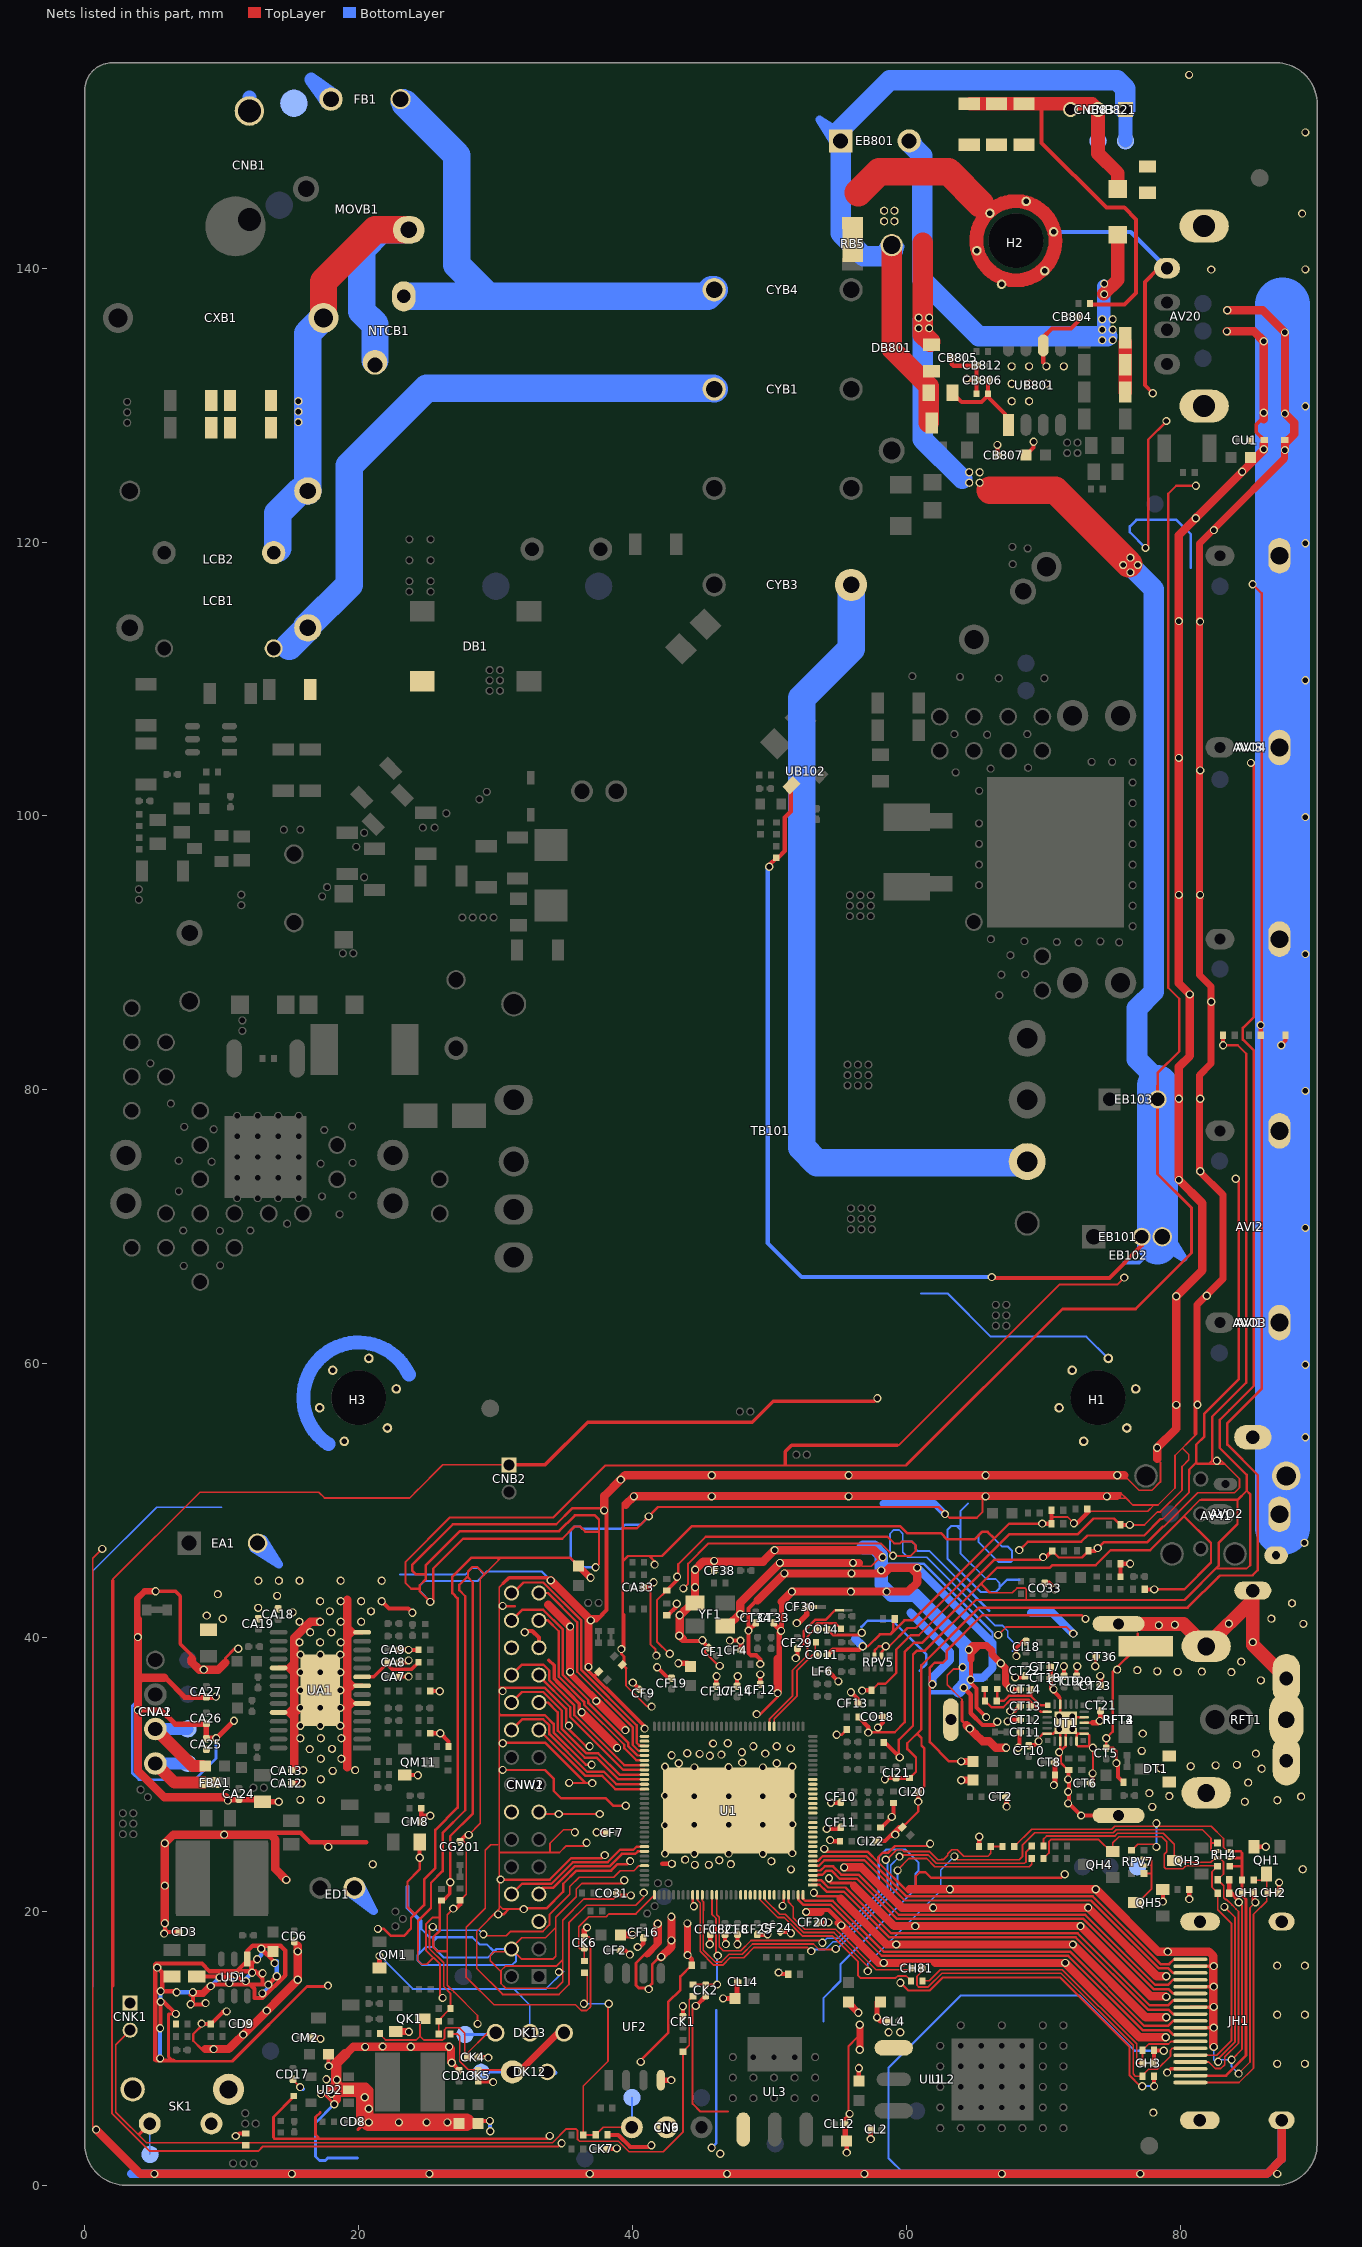
[diagram p0: the nets of this part, all layers, seen from the top]
# Altium PCB MISC116569.PcbDoc (part 10 of 15)
Units mm, origin at the board's own origin, x right, y up, seen from the top; angles counter-clockwise.
Board outline 90 x 155 mm, 2 copper layers (TopLayer, BottomLayer), stack 1.571 mm thick; 527 components, 277 nets, 2450 pads, 649 vias.

## Via types
v1: diameter 0.6, hole 0.4, TopLayer to BottomLayer, tented both sides, 649 vias

## Nets (pads, with @x,y where several pads share a name; then routed paths per layer and width w, separated by ;. In a path a pad name is that pad's centre, name@x,y a point inside that pad or via, vN(x,y) a via of type N, cw(c..) or ccw(c..) an arc to the next point about the centre after c; other vN are vias at no path point) (continued)
GND: (continued)
  BottomLayer w0.254: 23.546,21.78 23.546,20.255 24.385,19.416 24.385,16.989 ; v1(79.039,8.223) v1@79.039,8.295 ; v1@82.431,14.531 v1(82.456,14.506) ; v1(82.456,16.004) v1@82.456,16.035
  BottomLayer w0.3: v1(49.987,96.291) 49.873,96.178 49.873,68.803 52.357,66.319 v1(66.23,66.319) ; 75.946,67.373 76.98,67.373 EB102.2@78.349,68.742
  BottomLayer w0.305: v1@5.299,15.871 v1(5.299,15.89) ; v1(5.494,9.258) 5.498,9.262 v1(5.498,11.468) ; v1(5.532,14.16) 5.536,14.156 v1(5.536,13.399) ; v1(6.701,14.097) v1(7.895,14.097) ; v1@8.485,11.805 v1(8.526,11.805) ; v1(9.203,14.541) v1(9.838,15.176) ; v1(10.358,12.687) v1@10.473,12.687 ; v1(10.549,14.757) 10.652,14.655 10.652,14.975 v1(11.031,15.354) ; v1(11.755,14.91) 11.755,15.064 v1(12.214,15.523) ; v1(12.581,16.497) 12.917,16.834 12.917,17.241 v1(12.886,17.272) ; v1(12.975,14.008) 13.413,14.446 v1(13.413,14.649) ; v1(13.295,12.756) v1@13.324,12.756 ; v1(13.864,16.218) 14.022,16.377 v1(14.022,15.259) ; v1(15.548,15.009) 15.553,15.013 v1(15.553,17.069) ; v1@15.794,7.175 v1@15.938,7.031 ; v1(17.813,8.7) v1@17.851,8.661 ; v1(20.745,4.585) v1(20.745,5.577) ; 21.611,4.585 v1(22.944,4.585) ; v1(21.75,10.13) 21.77,10.109 v1(23.808,10.109) ; v1@23.63,39.091 v1(23.643,39.091) ; 24.201,4.585 v1(24.963,4.585) ; 25.725,4.585 v1(26.487,4.585) ; v1@25.903,36.068 v1(25.916,36.081) ; v1(26.805,8.943) v1@26.83,8.918 ; v1(29.591,4.699) 29.591,3.962 v1(29.616,3.937) ; v1@29.708,7.529 v1@29.737,7.529 ; DK12.K@34.334,8.238 DK12.K@34.359,8.213 ; v1(40.013,36.705) v1@40.089,36.629 ; v1(44.023,16.808) v1@44.1,16.731 ; v1@45.206,39.77 v1@45.238,39.77 ; v1(45.639,17.605) v1@45.664,17.63 ; v1@45.956,45.579 v1(45.956,45.593) ; v1@46.136,37.101 v1(46.136,37.169) ; v1@46.732,17.605 v1(46.824,17.605) ; v1@47.633,17.63 v1(47.658,17.605) ; v1@47.683,37.099 v1(47.683,37.169) ; v1@49.335,37.925 v1(49.335,38.064) ; v1@49.847,18.332 v1(49.863,18.332) ; v1(50.668,15.535) v1@50.757,15.623 ; v1@51.562,18.409 v1(51.567,18.404) ; v1@54.26,19.232 v1(54.3,19.192) ; v1(54.496,27.927) v1@54.514,27.927 ; v1(58.928,26.899) v1@58.928,26.924 ; v1(60.871,28.016) v1@60.884,28.003 ; 64.448,39.461 64.498,39.461 ; v1(66.632,33.848) v1@66.657,33.873 ; v1@67.584,36.274 v1@67.648,36.274 ; v1@70.738,36.219 v1(70.754,36.219) ; H2.4@70.75,142.654 76.386,142.654 AV20.4@79.04,140 ; v1(71.505,37.897) v1@71.533,37.925 ; v1@72.436,37.899 v1@72.449,37.887 ; v1@72.474,37.887 v1(72.487,37.899) ; v1@76.309,48.212 v1(76.322,48.224) ; v1(78.735,20.716) v1@78.748,20.729 ; v1(80.653,20.894) v1@80.653,20.97 ; v1(83.129,83.251) v1@83.155,83.251 ; v1(84.277,20.663) v1@84.346,20.663 ; v1(85.491,20.653) v1@85.504,20.665 ; v1(85.872,84.724) v1@85.897,84.7
  BottomLayer w0.33: 61.85,35.986 63.508,35.986
  BottomLayer w0.381: v1@9.58,35.602 v1(9.58,35.689) ; v1@15.799,29.362 v1(15.862,29.362) ; v1@21.509,16.726 v1(21.522,16.739) ; v1@36.588,18.821 v1(36.68,18.821) ; v1(46.617,13.642) v1@46.655,13.68 ; v1@52.002,41.036 v1(52.002,41.049) ; v1(67.318,27.648) v1@67.318,27.711 ; v1(74.155,37.189) v1@74.176,37.169
  BottomLayer w0.508: v1@23.655,11.214 v1(23.668,11.214) ; v1(45.779,2.743) v1@45.782,2.743 ; 58.306,49.784 62.05,49.784 v1(62.822,49.012)
  BottomLayer w0.61: 3.373,0.826 47.353,0.826 ; 47.816,0.826 47.353,0.826 ; 56.261,39.914 v1(56.815,39.36) ; v1@58.166,45.083 60.803,45.083 66.289,39.596 66.289,37.782 65.561,37.053 64.593,37.053 64.359,37.287 ; 60.308,41.806 63.173,38.941 63.173,38.356 61.908,37.091 v1(61.908,36.591) ; 69.121,41.819 70.65,41.819 v1(72.182,40.287) ; JH1.21@87.409,4.75 87.409,1.907 86.327,0.826 47.353,0.826
  BottomLayer w1: pad.VIA5@74.417,135.255 pad.VIA5@74.417,138.659
  BottomLayer w1.016: 17.786,54.12 cw(c20,57.502) 23.667,59.204 ; 56.87,46.581 57.623,46.581 58.166,46.039 58.166,43.867 58.927,43.106 60.624,43.106 63.803,39.927 ; 63.826,36.136 64.359,36.669 64.359,39.372 63.803,39.927 ; 64.185,39.545 63.803,39.927
  BottomLayer w1.5: EB801.2@60.242,149.119 61.149,148.212 61.149,144.412 ; 61.149,139.201 61.149,140.437 ; 61.149,145.907 61.149,144.412 ; 61.209,136.195 61.209,127.495 64.079,124.625 ; 74.658,135.026 65.291,135.026 61.149,139.168 61.149,140.437 ; 76.233,118.402 78.067,116.568 78.067,87.165 76.843,85.941 76.843,82.233 78.177,80.898 78.177,80.675 78.443,80.409 ; 61.149,140.437 61.149,144.412
  BottomLayer w2: CYB3.2@55.964,116.874 55.964,112.212 52.362,108.61 52.362,75.789 53.473,74.678 TB101.8@68.643,74.678
  BottomLayer w3: EB102.2@78.349,68.742 78.349,80.315
  BottomLayer w4: AVO3.2@87.479,48.012 87.479,54.892 ; 87.479,52.9 87.479,54.892 ; 87.479,137.34 87.479,54.892
  other v1: 5.088,0.826 15.126,0.826 25.172,0.826 36.881,0.826 46.901,0.826 56.939,0.826 66.98,0.826 77.077,0.826 87.084,0.826 46.414,2.294 29.813,7.529 58.701,11.178 59.56,11.178 78.983,12.264 55.248,18.976 42.845,19.599 30.201,19.773 44.488,20.372 44.524,24.207 49.524,24.207 42.374,24.219 47.012,24.219 51.674,24.257 42.374,26.282 44.524,26.307 49.524,26.307 47.012,26.319 51.674,26.357 71.814,27.879 44.524,28.407 47.012,28.419 49.524,28.407 42.374,28.457 51.674,28.457 71.814,28.743 71.814,29.632 44.524,30.507 49.524,30.507 47.012,30.519 42.374,30.557 51.674,30.557 50.533,30.811 48.01,30.866 45.656,31.37 42.858,31.394 46.495,31.446 44.894,31.501 49.695,31.522 44.005,31.548 51.549,31.903 48.831,32.056 77.262,32.982 71.157,33.297 72.107,33.297 15.754,33.554 17.204,33.554 18.654,33.554 71.157,34.247 72.107,34.247 15.754,34.854 17.204,34.854 18.654,34.854 15.754,36.154 17.204,36.154 18.654,36.154 15.754,37.454 17.204,37.454 18.654,37.454 8.687,37.655 15.754,38.754 17.204,38.754 18.654,38.754 10.071,41.377 8.903,41.605 36.939,44.364 56.104,45.443 55.784,50.305 45.783,51.854 55.784,51.854 65.784,51.854 89.147,54.625 89.147,59.913 89.147,69.913 89.147,79.913 82.261,86.436 89.147,89.913 81.448,94.234 89.147,99.913 79.904,104.234 89.147,109.913 81.453,114.191 79.904,114.234 89.147,119.913 86.101,126.771 89.147,129.913 82.271,139.9 89.147,139.913 88.9,143.993 89.147,149.913 80.645,154.12
GVDD: CA8.2@22.114,38.177 CA8.2@22.289,38.177 RA10.1 UA1.9 | length 5
  TopLayer w0.254: UA1.9@20.254,37.129 21.092,37.129 22.114,38.151 22.114,37.993 22.409,37.698 23.888,37.698 24.379,38.189 RA10.1@24.379,38.195
HDMI_A_0N_IN_IC: JH1.9 U1.1 | length 32.3
  TopLayer w0.178: U1.1@53.075,21.932 U1.1@53.175,21.932 53.672,21.932 54.166,21.438 55.425,21.438 58.764,18.1 72.376,18.1 77.649,12.827 79.154,12.827 ; 78.392,12.827 79.154,12.827 ; JH1.9@80.742,12.5 79.481,12.5 79.154,12.827
HDMI_A_0P_IN_IC: JH1.7 U1.2 | length 31.5
  TopLayer w0.178: U1.2@53.175,22.282 53.753,22.282 54.292,21.743 55.551,21.743 58.89,18.405 72.502,18.405 77.775,13.131 79.103,13.131 79.472,13.5 JH1.7@80.742,13.5
HDMI_A_1N_IN_IC: JH1.6 U1.3 | length 31.4
  TopLayer w0.178: U1.3@53.175,22.632 53.526,22.632 53.571,22.678 53.868,22.678 54.167,22.977 54.522,22.977 55.12,22.378 56.389,22.378 59.321,19.446 72.933,19.446 78.053,14.327 79.154,14.327 79.481,14 JH1.6@80.742,14
HDMI_A_1P_IN_IC: JH1.4 U1.4 | length 31.4
  TopLayer w0.178: U1.4@53.175,22.982 53.741,22.982 54.041,23.282 54.648,23.282 55.247,22.683 56.515,22.683 59.448,19.751 73.059,19.751 78.179,14.631 79.103,14.631 79.472,15 JH1.4@80.742,15
HDMI_A_2N_IN_IC: JH1.3 U1.5 | length 31.1
  TopLayer w0.178: U1.5@53.175,23.332 53.619,23.332 54.019,23.732 56.939,23.732 59.879,20.792 73.491,20.792 78.446,15.837 79.144,15.837 79.481,15.5 JH1.3@80.742,15.5
HDMI_A_2P_IN_IC: JH1.1 U1.6 | length 31.1
  TopLayer w0.178: U1.6@53.175,23.682 53.538,23.682 53.893,24.037 57.065,24.037 60.005,21.097 73.617,21.097 78.572,16.142 79.19,16.142 79.548,16.5 JH1.1@80.742,16.5
HDMI_A_5V: CH1.1 JH1.18 RH3.2 RH4.1 RH4.3 RH4.5 RH81.2 RPV7.1 | length 44.4
  TopLayer w0.127: RH81.2@67.881,24.74 69.145,26.003 75.002,26.003 75.214,26.215 82.271,26.215 83.163,25.323 83.163,24.684 83.453,24.394 RH4.5@83.622,24.394 ; RPV7.1@76.451,24.458 76.891,24.898 78.198,24.898 78.265,24.831 v1(78.265,24.704) ; v1@78.252,26.418 v1(78.265,26.431)
  TopLayer w0.203: JH1.18@80.742,8 83.34,8 84.806,9.466 84.806,20.882 84.52,21.167 CH1.1@84.52,21.365 ; RH4.1@83.622,23.294 84.52,23.294 ; RH4.3@83.622,23.894 84.52,23.894 ; RH4.5@83.622,24.394 84.391,24.394 84.52,24.265 84.52,23.894 ; CH1.1@84.608,21.277 CH1.1@84.52,21.365 ; CH1.1@84.52,21.365 RH3.2@84.52,22.278 84.52,23.294 ; 84.52,23.294 84.52,23.894
  BottomLayer w0.127: v1(78.265,24.704) 78.265,25.479 ; 78.265,26.05 78.265,25.479 ; v1(78.265,26.431) 78.265,25.479
HDMI_A_CKN_IN_IC: JH1.12 U1.127 | length 33.1
  TopLayer w0.178: U1.127@52.099,21.207 52.099,20.854 52.48,20.473 54.487,20.473 58.206,16.754 71.818,16.754 77.245,11.327 79.154,11.327 79.481,11 JH1.12@80.742,11
HDMI_A_CKP_IN_IC: JH1.10 U1.128 | length 33.3
  TopLayer w0.178: U1.128@52.449,21.207 52.449,20.935 52.606,20.778 54.613,20.778 58.332,17.059 71.944,17.059 77.371,11.631 79.103,11.631 ; 78.392,11.631 79.103,11.631 ; JH1.10@80.742,12 79.472,12 79.103,11.631
HDMI_A_HPD_OUT: CH2.1 JH1.19 QH1.C RH3.1 | length 21.1
  TopLayer w0.127: JH1.19@80.742,7.5 84.297,7.5 85.352,8.554 85.352,19.776 86.317,20.742 QH1.C@86.317,22.735 QH1.C@86.59,22.461 ; RH3.1@85.37,22.278 QH1.C@86.408,22.278
HDMI_A_HPD_OUT_IC: RH4.6 RH4.8 U1.120 | length 44.4
  TopLayer w0.127: U1.120@49.649,21.207 49.698,21.157 49.698,20.829 50.743,19.784 51.168,19.784 52.504,18.448 54.716,18.448 57.188,15.976 v1(57.188,15.642) ; U1.120@49.649,21.207 U1.120@49.65,21.257 ; v1(63.513,24.016) 63.754,23.774 64.668,23.774 ; 63.856,23.774 64.668,23.774 ; RH4.6@82.722,24.394 82.334,24.394 82.245,24.483 82.245,24.996 ; RH4.8@82.722,24.994 82.72,24.996 82.245,24.996 ; 64.668,23.774 68.247,23.774 68.489,24.016 68.489,24.853 69.385,25.749 75.107,25.749 75.319,25.961 81.631,25.961 82.245,25.347 82.245,24.996
  BottomLayer w0.127: v1(57.188,15.642) 57.188,16.194 62.517,21.524 62.517,23.02 v1(63.513,24.016)
HDMI_A_SCL_IN: DH2.K JH1.15 QH4.E RH4.2 RH6.1 | length 34.3
  TopLayer w0.127: RH6.1@70.008,23.863 70.409,24.264 70.409,25.095 70.555,25.241 74.047,25.241 74.917,24.371 QH4.E@75.082,24.371 75.082,25.006 75.529,25.453 78.659,25.453 79.018,25.094 79.018,24.366 78.832,24.18 78.832,23.222 78.944,23.11 80.201,23.11 80.417,23.326 82.691,23.326 RH4.2@82.722,23.294 82.321,22.893 82.321,21.754 DH2.K@82.736,21.338 82.736,20.122 83.752,19.107 83.752,10.582 82.67,9.5 JH1.15@80.742,9.5
HDMI_A_SCL_IN_IC: RH6.2 U1.107 | length 33.4
  TopLayer w0.127: U1.107@45.099,21.207 45.1,20.785 45.183,20.702 45.183,20.064 ; 45.174,20.055 45.174,17.169 46.039,16.304 46.493,16.304 47.049,16.86 48.01,16.86 48.763,17.613 53.221,17.613 53.622,17.213 54.804,17.213 v1(54.851,17.26) ; v1@59.36,23.046 60.173,23.858 61.489,23.858 62.081,23.266 68.984,23.266 69.158,23.441 RH6.2@69.158,23.863
  BottomLayer w0.127: v1(54.851,17.26) 54.944,17.26 59.36,21.675 v1(59.36,22.987)
HDMI_A_SDA_IO: DH3.K JH1.16 QH3.C RH4.4 RH5.1 | length 34.4
  TopLayer w0.127: RH5.1@70.008,24.778 70.008,25.266 70.237,25.495 75.212,25.495 75.424,25.707 78.764,25.707 79.018,25.453 ; JH1.16@80.742,9 82.082,9 82.563,8.519 82.969,8.519 83.257,8.806 83.257,9.368 84.26,10.371 84.26,19.986 84.074,20.172 83.787,20.459 83.373,20.873 83.283,20.873 83.171,20.984 83.171,21.869 DH3.K@82.736,22.304 83.163,22.73 83.163,23.623 RH4.4@82.892,23.894 ; RH4.4@82.722,23.894 82.553,23.894 82.239,23.58 79.693,23.58 QH3.C@79.572,23.701 79.572,24.899 79.027,25.444 ; 79.018,25.453 79.027,25.444 ; 79.018,25.453 79.027,25.453 79.027,25.444
HDMI_A_SDA_IO_IC: RH5.2 U1.106 | length 34.9
  TopLayer w0.127: U1.106@44.749,21.207 44.75,20.812 44.954,20.607 44.954,20.159 ; U1.106@44.749,21.207 U1.106@44.759,21.198 ; 44.945,20.149 44.945,17.075 45.944,16.075 46.587,16.075 47.118,16.606 48.115,16.606 48.868,17.359 52.782,17.359 v1(53.047,17.094) ; v1(59.499,24.003) 59.609,24.112 61.595,24.112 62.187,23.52 68.628,23.52 68.743,23.635 68.743,24.362 RH5.2@69.158,24.778
  BottomLayer w0.127: v1@53.047,17.174 52.967,17.174 v1(53.047,17.094) 53.165,17.213 54.069,17.213 54.642,17.785 55.11,17.785 58.869,21.544 58.869,23.373 v1(59.499,24.003)
HDMI_ARC_OUT: CH81.1 DH81.K JH1.14 | length 27.3
  TopLayer w0.127: CH81.1@61.19,15.839 61.19,15.683 60.774,15.268 60.774,14.596 60.887,14.483 61.601,14.483 62.602,15.484 71.292,15.484 76.563,10.212 76.563,8.13 76.728,7.965 77.186,7.965 77.685,8.465 78.327,8.465 79.289,9.426 79.289,9.866 79.424,10 JH1.14@80.742,10
HDMI_ARC_OUT_IC: CH81.2@60.34,15.839 CH81.2@60.515,15.839 U1.125 | length 12
  TopLayer w0.127: U1.125@51.399,21.207 51.399,20.664 51.748,20.316 51.748,19.528 52.574,18.702 54.821,18.702 55.245,18.278 57.785,15.738 60.238,15.738 CH81.2@60.34,15.839
HDMI_B_0N_IN_IC: U1.9
HDMI_B_0P_IN_IC: U1.10
HDMI_B_1N_IN_IC: U1.11
HDMI_B_1P_IN_IC: U1.12
HDMI_B_2N_IN_IC: U1.13
HDMI_B_2P_IN_IC: U1.14
HDMI_B_CKN_IN_IC: U1.7
HDMI_B_CKP_IN_IC: U1.8
HDMI_B_HPD_OUT_IC: U1.121
HDMI_B_SCL_IN_IC: U1.116
HDMI_B_SDA_IO_IC: U1.115
HDMI_C_0N_IN_IC: U1.18
HDMI_C_0P_IN_IC: U1.19
HDMI_C_1N_IN_IC: U1.20
HDMI_C_1P_IN_IC: U1.21
HDMI_C_2N_IN_IC: U1.22
HDMI_C_2P_IN_IC: U1.23
HDMI_C_CKN_IN_IC: U1.16
HDMI_C_CKP_IN_IC: U1.17
HDMI_C_HPD_OUT_IC: U1.122
HDMI_C_SCL_IN_IC: U1.118
HDMI_C_SDA_IO_IC: U1.117
HDMI_CEC_IO: CH3.2@77.239,8.905 CH3.2@77.414,8.905 DH1.K JH1.13 RH83.2 | length 24.7
  TopLayer w0.127: RH83.2@61.19,14.925 61.669,14.925 62.481,15.738 71.397,15.738 76.817,10.317 76.817,8.981 76.894,8.905 CH3.2@77.239,8.905 77.239,9.841 DH1.K@77.243,9.845 77.709,10.311 79.144,10.311 79.333,10.5 JH1.13@80.742,10.5
HDMI_CEC_IO_IC: RH83.1 U1.119 | length 14.6
  TopLayer w0.127: U1.119@49.3,21.257 49.3,21.207 49.299,20.87 50.624,19.545 ; 50.631,19.552 51.076,19.552 52.435,18.194 54.611,18.194 56.473,16.332 56.473,16.296 ; 56.473,16.296 56.473,15.309 56.642,15.14 59.232,15.14 59.368,15.276 59.989,15.276 RH83.1@60.34,14.925
HDMI_DET: RH81.1 RH82.1 U1.110 | length 30.4
  TopLayer w0.127: U1.110@46.15,21.207 46.15,19.757 46.333,19.573 46.333,17.402 46.622,17.114 47.904,17.114 48.657,17.867 v1@53.702,17.867 ; v1@58.49,23.831 v1(58.49,23.773) 58.576,23.773 59.296,24.493 59.703,24.493 59.83,24.366 61.7,24.366 62.292,23.774 62.56,23.774 62.565,23.779 62.7,23.779 63.022,24.102 63.022,24.219 63.31,24.506 63.716,24.506 64.194,24.028 65.964,24.028 66.167,24.232 RH82.1@66.167,24.74 RH81.1@67.032,24.74
  BottomLayer w0.127: v1(53.866,17.703) 54.202,18.039 55.005,18.039 58.615,21.649 v1@58.615,23.648
I2C_EN: QH5.C RPV7.4 RPV7.6 RPV7.8 | length 5.4
  TopLayer w0.127: QH5.C@76.753,20.64 76.894,20.64 77.91,21.656 77.91,22.748 ; RPV7.8@77.351,22.758 77.9,22.758 77.91,22.748 ; RPV7.6@77.351,23.358 77.871,23.358 77.91,23.396 ; RPV7.4@77.351,23.858 77.778,23.858 77.91,23.726 77.91,23.396 ; 77.91,22.748 77.91,23.396
IF_N: CT13.1 RT10.1 RT12.2 UT1.14 | length 6.3
  TopLayer w0.178: RT12.2@65.711,35.407 RT10.1@65.711,36.263 ; RT12.2@65.75,35.368 66.216,34.902 67.077,34.902 67.619,35.444 68.948,35.444 69.82,34.572 UT1.14@70.282,34.572 ; CT13.1@68.933,34.978 CT13.1@69.108,34.978
IF_P: CT14.2@68.94,36.21 CT14.2@69.115,36.21 RT12.1 RT13.1 UT1.13 | length 5.5
  TopLayer w0.178: RT13.1@66.651,36.263 66.651,35.419 RT12.1@66.6,35.368 67.112,35.368 67.492,35.749 69.074,35.749 ; CT14.2@69.115,36.185 69.115,35.789 69.074,35.749 ; UT1.13@70.336,35.067 69.756,35.067 69.074,35.749
IR_IN: CN6.1 CN9.1 DK3.K IR_IN.1 RK12.1 RK19.1 | length 20.8
  TopLayer w0.127: v1(36.457,13.249) 36.69,13.249 36.703,13.261 36.703,15.295 RK19.1@36.482,15.516 ; v1(38.26,13.249) 38.209,13.198 38.209,9.045 36.406,7.241 RK12.1@36.406,3.673 DK3.K@37.314,3.673 37.868,4.227 CN9.1@39.954,4.227
  BottomLayer w0.127: v1(36.457,13.249) v1(38.26,13.249) v1@38.209,13.299 ; CN9.1@39.962,4.234 IR_IN.1@39.962,6.403
IR_IN_IC: CK6.2@36.482,17.294 CK6.2@36.482,17.469 RK19.2 U1.97 | length 9.4
  TopLayer w0.127: RK19.2@36.482,16.366 CK6.2@36.482,17.294 36.133,17.294 36.067,17.359 36.067,18.866 36.816,19.615 38.083,19.615 38.28,19.812 40.248,19.812 41.599,21.163 U1.97@41.599,21.207
K0: CNK1.2 DK1.K K0.1 RK3.2 RK4.1 SK1.2 | length 65.7
  TopLayer w0.127: CNK1.2@3.31,11.319 2.261,10.27 2.261,5.34 4.502,3.099 34.161,3.099 35.175,4.113 35.86,4.113 35.99,3.983 35.99,3.344 36.131,3.203 38.981,3.203 39.746,2.438 42.246,2.438 43.683,3.876 RK4.1@43.683,9.75 44.153,10.22 44.153,12.855 ; 44.153,11.565 44.153,12.855 ; RK3.2@44.42,13.801 44.153,13.535 44.153,12.855
  TopLayer w0.254: 3.979,3.712 3.979,3.732 SK1.2@4.746,4.5
  BottomLayer w0.127: K0.1@4.746,2.274 SK1.2@4.746,4.5
KEY_IN_IC: CK2.1 RK3.1 U1.109 | length 8.5
  TopLayer w0.127: RK3.1@44.42,14.651 CK2.1@45.347,14.651 ; 45.08,14.658 v1(46.172,14.658) ; U1.109@45.8,21.207 45.8,19.783 46.105,19.478 v1@46.105,16.896
  BottomLayer w0.127: v1(46.172,14.658) v1@46.172,16.71
  other v1: 46.232,16.769
L: CYB1.1 DB1.2 LCB1.4 LCB2.4@16.293,113.731 RB101.1 | length 44
  BottomLayer w2: 14.943,112.381 LCB2.4@16.293,113.731 ; LCB2.4@16.222,113.802 19.306,116.886 19.306,125.561 24.985,131.24 45.899,131.24 CYB1.1@45.964,131.176
L-1: CNB1.1 FB1.1 TP_L.1 | length 1.4
  BottomLayer w1: CNB1.1@12.023,151.484 CNB1.1@12.023,152.471 ; FB1.1@17.549,152.348 FB1.1@17.98,152.348
L-2: CXB1.1 LCB1.1 LCB2.1 MOVB1.1 NTCB1.1 pad.VIA5@15.603,128.765 pad.VIA5@15.603,129.527 pad.VIA5@15.603,130.289 RB1.1 RB2.1 | length 41.5
  TopLayer w2: CXB1.1@17.431,136.373 17.431,139.013 21.215,142.797 MOVB1.1@23.659,142.797
  BottomLayer w2: LCB1.1@14.106,119.544 14.106,122.094 15.743,123.731 LCB2.1@16.293,123.731 16.293,135.234 CXB1.1@17.431,136.373 ; NTCB1.1@21.194,133.261 21.194,135.9 20.226,136.868 20.226,141.402 21.623,142.799 MOVB1.1@23.657,142.799
L-5: CYB4.1 FB1.2 NTCB1.2@23.295,137.947 | length 39.8
  BottomLayer w2: FB1.2@23.391,152.016 27.173,148.234 27.173,140.246 29.472,137.947 ; NTCB1.2@23.668,137.947 29.472,137.947 ; CYB4.1@45.789,138.428 CYB4.1@45.308,137.947 ; CYB4.1@45.964,138.428 45.483,137.947 CYB4.1@45.308,137.947 ; 29.472,137.947 CYB4.1@45.308,137.947
L-N: RB1.2 RB2.2 RB3.1 RB4.1
LED+: CB808.2 CB811.2 CNB821.1 CNB831.1 DB801.K EB801.1@55.204,149.299 RB812.2 RB814.2 TP_LED+.1 | length 52.7
  TopLayer w1.5: DB801.K@58.929,141.708 58.929,134.093 60.149,132.874 61.639,131.384 RB814.2@61.639,130.899 61.639,129.781 RB812.2@61.639,128.727
  BottomLayer w1: TP_LED+.1@76.002,149.305 CNB821.1@76.002,151.591
  BottomLayer w1.5: EB801.1@55.204,149.119 EB801.1@55.204,149.299 ; 58.929,140.868 58.513,140.868 56.874,140.868 55.204,142.538 EB801.1@55.204,149.299 ; CNB821.1@76.002,151.591 76.002,153.117 75.387,153.732 58.794,153.732 55.204,150.141 55.204,149.882 EB801.1@55.204,149.299
LED_FB: CB808.1 CNB821.2 CNB831.2 CNB831.3 DB804.A RB805.2 RB837.2 RB838.2 RB839.1 TP_LED-.1 | length 39.3
  TopLayer w0.3: 69.782,151.923 69.875,151.83 69.875,149.157 74.608,144.424 75.916,144.424 76.779,143.561 76.779,138.197 75.939,137.356 73.482,137.356 RB805.2@73.412,137.427
  TopLayer w1: RB837.2@64.689,152.012 73.581,152.012 CNB821.2@74.002,151.591 74.002,148.375 75.433,146.944 DB804.A@75.433,145.795
  BottomLayer w1: TP_LED-.1@74.002,149.305 CNB821.2@74.002,151.591
LED_G: CK4.1 DK13.1 LED_G.1 QK1.C RK10.1 | length 15.5
  TopLayer w0.127: RK10.1@21.636,10.937 21.969,10.604 24.201,10.604 24.483,10.886 ; QK1.C@24.659,12.017 24.483,11.841 24.483,10.886 ; DK13.1@30.003,11.129 29.422,11.129 27.916,9.623 CK4.1@27.916,9.362 27.745,9.534 27.745,11.09 27.342,11.492 26.399,11.492 26.269,11.361 26.269,10.723 26.151,10.604 24.765,10.604 24.483,10.886
  BottomLayer w0.203: LED_G.1@27.764,11.001 DK13.1@29.874,11.001
LED_OUT_IC: RK13.1 RK14.1 RK15.2 U1.92 | length 27.6
  TopLayer w0.127: v1(25.417,18.865) 25.171,18.619 25.171,17.275 26.213,16.234 26.213,14.508 26.703,14.017 RK15.2@26.703,12.906 ; RK14.1@25.853,11.051 RK13.1@25.853,11.979 25.853,12.056 RK15.2@26.703,12.906 ; RK15.2@26.563,13.045 RK15.2@26.703,12.906 ; v1@29.235,18.209 30.787,18.209 31.114,18.536 33.46,18.536 33.933,19.01 33.933,19.75 35.426,21.242 35.426,21.818 36.102,22.494 38.638,22.494 39.116,22.972 40.108,22.972 40.468,23.332 U1.92@40.873,23.332 ; U1.92@40.875,23.332 U1.92@40.925,23.332
  BottomLayer w0.127: v1(25.417,18.865) 25.508,18.865 25.744,18.629 28.816,18.629 v1(29.116,18.329) v1@29.116,18.31
LED_OVP: CB806.1 RB803.2 RB814.1 UB801.1 | length 6.2
  TopLayer w0.305: RB814.1@63.371,130.899 64.04,130.23 65.487,130.23 RB803.2@65.965,130.707 ; RB803.2@65.965,130.835 RB803.2@65.965,130.708 ; CB806.1@65.965,131.826 RB803.2@65.965,130.707 ; UB801.1@67.21,129.343 65.965,130.588 RB803.2@65.965,130.707
LED_R: CK5.1 DK12.A DK13.3 LED_R.1 RK14.2 | length 14
  TopLayer w0.127: RK14.2@26.703,11.051 27.198,11.051 27.376,10.874 27.376,9.065 28.017,8.425 28.017,8.416 CK5.1@28.735,8.416 31.093,8.416 DK12.A@31.235,8.274
  TopLayer w0.508: DK12.A@31.235,8.274 31.711,8.274 34.566,11.129 DK13.3@35.003,11.129
  BottomLayer w0.203: LED_R.1@28.951,8.245 DK12.A@31.206,8.245
LINE_L_OUT_IC: CO11.2@53.41,38.735 CO11.2@53.585,38.735 RO12.1 U1.39 | length 7.5
  TopLayer w0.127: U1.39@50.349,33.508 50.349,34.068 52.019,35.738 52.019,37.603 53.151,38.735 CO11.2@53.41,38.735 ; CO11.2@53.337,38.808 53.355,38.826 RO12.1@53.355,39.652
LINE_R_OUT_IC: CO14.2@53.393,40.592 CO14.2@53.568,40.592 RO15.1 U1.40 | length 10.8
  TopLayer w0.127: U1.40@49.999,33.508 49.999,34.041 51.679,35.722 51.679,37.587 52.774,38.682 52.774,40.065 CO14.2@53.301,40.592
  TopLayer w0.178: CO14.2@53.393,40.592 53.393,40.941 53.483,41.032 54.832,41.032 RO15.1@55.221,40.642
LOUT+: CNA1.4 CNA2.4 FBA1.2 FBA1.3 LOUT+.1 | length 6.5
  TopLayer w0.889: CNA1.4@5.156,30.795 6.551,29.4 FBA1.2@8.725,29.4
  BottomLayer w0.889: CNA1.4@5.156,30.795 7.51,30.795 LOUT+.1@7.526,30.811
LOUT-: BA2.2 CA25.1 CNA1.3 CNA2.3 LOUT-.1 | length 7.9
  TopLayer w0.762: CNA1.3@5.156,33.315 CNA1.3@5.55,33.315
  TopLayer w0.889: CNA1.3@5.594,32.877 CNA1.3@5.156,33.315 7.864,30.607 BA2.2@8.598,30.607
  BottomLayer w0.889: CNA1.3@5.156,33.315 LOUT-.1@7.51,33.315
LVDS_E0N_IC: CNW1.19 CNW2.19 U1.76 | length 9.5
  TopLayer w0.178: CNW2.19@33.164,33.251 33.193,33.251 36.556,29.889 37.788,29.889 38.744,28.932 U1.76@40.873,28.932 U1.76@40.875,28.932
LVDS_E0P_IC: CNW1.20 CNW2.20 U1.75 | length 12.4
  TopLayer w0.178: CNW2.20@31.164,33.251 31.93,34.017 33.481,34.017 33.93,33.569 33.93,32.946 36.682,30.193 37.914,30.193 38.825,29.282 U1.75@40.873,29.282 U1.75@40.875,29.282
LVDS_E1N_IC: CNW1.21 CNW2.21 U1.74 | length 12
  TopLayer w0.178: CNW2.21@33.164,35.197 CNW2.21@33.164,35.251 33.816,35.251 34.539,34.528 34.539,33.821 34.539,33.199 36.511,31.227 37.377,31.227 38.971,29.632 U1.74@40.873,29.632 ; 39.748,29.632 U1.74@40.875,29.632
LVDS_E1P_IC: CNW1.22 CNW2.22 U1.73 | length 14.4
  TopLayer w0.178: CNW2.22@31.164,35.251 31.93,36.017 33.481,36.017 34.844,34.654 34.844,33.325 36.637,31.532 37.503,31.532 39.052,29.982 U1.73@40.873,29.982 ; 39.829,29.982 U1.73@40.873,29.982 ; U1.73@40.875,29.982 U1.73@40.873,29.982
LVDS_E2N_IC: CNW1.23 CNW2.23 U1.72 | length 12
  TopLayer w0.178: CNW2.23@33.164,37.251 33.164,37.197 35.454,34.907 35.454,34.2 39.321,30.332 U1.72@40.873,30.332 ; 39.91,30.332 U1.72@40.873,30.332 ; U1.72@40.875,30.332 U1.72@40.873,30.332
LVDS_E2P_IC: CNW1.24 CNW2.24 U1.71 | length 14.8
  TopLayer w0.178: CNW2.24@31.164,37.251 31.93,38.017 33.481,38.017 33.93,37.569 33.93,36.862 35.758,35.033 35.758,34.326 39.402,30.682 U1.71@40.873,30.682 ; 39.991,30.682 U1.71@40.873,30.682 ; U1.71@40.875,30.682 U1.71@40.873,30.682
LVDS_E3N_IC: CNW1.29 CNW2.29 U1.68 | length 15.4
  TopLayer w0.178: CNW2.29@33.164,43.251 33.816,43.251 35.962,41.106 35.962,40.376 35.962,37.499 40.002,33.458 40.002,32.171 40.441,31.732 U1.68@40.873,31.732 ; U1.68@40.875,31.732 40.86,31.747 40.865,31.747 U1.68@40.875,31.756
LVDS_E3P_IC: CNW1.30 CNW2.30 U1.67 | length 17.8
  TopLayer w0.178: CNW2.30@31.225,43.19 32.053,44.017 33.481,44.017 36.266,41.232 36.266,37.626 40.307,33.585 40.307,32.297 40.498,32.106 40.849,32.106 U1.67@40.873,32.082 U1.67@40.875,32.082
LVDS_E4N_IC: U1.66
LVDS_E4P_IC: U1.65
LVDS_ECKN_IC: CNW1.27 CNW2.27 U1.70 | length 14.1
  TopLayer w0.178: CNW2.27@33.164,41.251 33.816,41.251 34.615,40.452 34.615,37.146 36.469,35.292 36.469,35.088 39.393,32.164 39.393,31.919 40.279,31.032 U1.70@40.873,31.032 U1.70@40.875,31.032
LVDS_ECKP_IC: CNW1.28 CNW2.28 U1.69 | length 16.7
  TopLayer w0.178: CNW2.28@31.164,41.251 31.93,42.017 33.481,42.017 34.92,40.578 34.92,37.272 36.774,35.418 36.774,35.214 39.698,32.29 39.698,32.045 40.36,31.382 U1.69@40.873,31.382 ; U1.69@40.849,31.406 U1.69@40.873,31.382 ; U1.69@40.875,31.382 U1.69@40.873,31.382
LVDS_O0N_IC: CNW1.7 CNW2.7 U1.89 | length 9.1
  TopLayer w0.178: CNW2.7@33.164,21.251 33.164,21.429 33.447,21.713 34.207,21.713 35.776,23.282 38.312,23.282 39.222,24.191 40.198,24.191 40.39,24.382 U1.89@40.873,24.382
LVDS_O0P_IC: CNW1.8 CNW2.8 U1.88 | length 11.2
  TopLayer w0.178: CNW2.8@31.164,21.251 31.93,22.017 34.081,22.017 35.65,23.586 38.186,23.586 39.095,24.496 40.072,24.496 40.309,24.732 U1.88@40.873,24.732